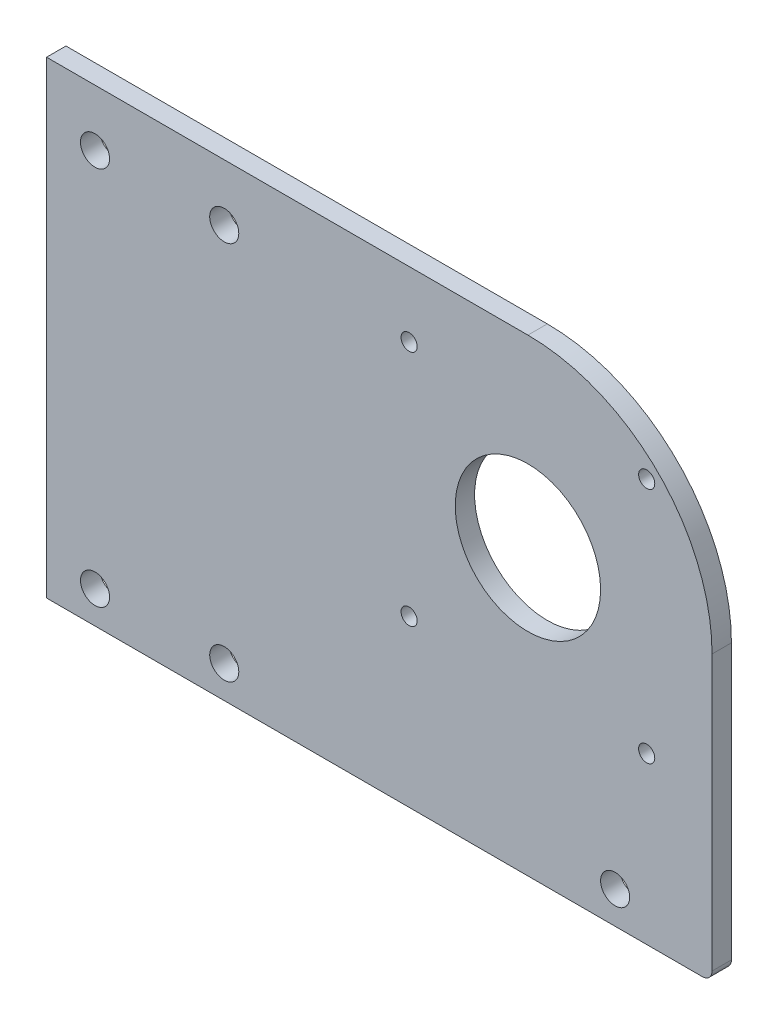
SolidWorks part; units mm, degrees
material "普通碳钢"
ref_plane "前视基准面" through (0, 0, 0) normal (0, 0, 1) x (1, 0, 0)
ref_plane "上视基准面" through (0, 0, 0) normal (0, 1, 0) x (1, 0, 0)
ref_plane "右视基准面" through (0, 0, 0) normal (1, 0, 0) x (0, 0, -1)
sketch "草图1" plane through (0, 0, 0) normal (0, 0, 1) x (1, 0, 0)
  line L0 (0, 72.5) -> (0, 0) construction
  line L1 (-103, 72.5) -> (103, 72.5)
  line L2 (-103, 72.5) -> (-103, -72.5)
  line L3 (-103, -72.5) -> (103, -72.5)
  line L4 (103, 72.5) -> (103, -72.5)
  line L5 (0, 0) -> (103, 0) construction
  dimension "D1" = 206
  dimension "D2" = 145
extrude "凸台-拉伸1" add sketch "草图1" along normal blind 6
sketch "草图2" plane through (0, 0, 6) normal (0, 0, 1) x (1, 0, 0)
  line L0 (103, 72.5) -> (-103, 72.5) construction
  line L1 (-103, -72.5) -> (-3, -72.5)
  line L2 (-103, -72.5) -> (-103, -7.5)
  line L3 (-103, -7.5) -> (-3, -7.5)
  line L4 (-3, -72.5) -> (-3, -7.5)
  dimension "D1" = 80
  dimension "D2" = 100
extrude "切除-拉伸1" [suppressed] cut sketch "草图2" against normal through all
sketch "草图3" plane through (0, 0, 6) normal (0, 0, 1) x (1, 0, 0)
  line L0 (103, 72.5) -> (-103, 72.5) construction
  line L1 (-103, 72.5) -> (-103, -72.5) construction
  circle A0 centre (-88, 55) radius 4.5
  circle A1 centre (-48, 55) radius 4.5
  circle A2 centre (-88, -62.5) radius 4.5
  circle A3 centre (-48, -62.5) radius 4.5
  dimension "D1" = 9
  dimension "D2" = 40
  dimension "D3" = 117.5
  dimension "D4" = 17.5
  dimension "D5" = 15
extrude "切除-拉伸2" cut sketch "草图3" against normal through all
sketch "草图4" plane through (0, 0, 6) normal (0, 0, 1) x (1, 0, 0)
  line L0 (103, 72.5) -> (-103, 72.5) construction
  line L2 (103, -72.5) -> (103, 72.5) construction
  circle A0 centre (46, 15.5) radius 22.5
  dimension "D1" = 45
  dimension "D3" = 57
  dimension "D2" = 57
extrude "切除-拉伸3" cut sketch "草图4" against normal through all
fillet "圆角1" radius 57 1 edges at (103, 72.5, 3)
fillet "圆角2" [suppressed] radius 10
fillet "圆角3" [suppressed] radius 10
sketch "草图5" plane through (0, 0, 6) normal (0, 0, 1) x (1, 0, 0)
  line L0 (46, 72.5) -> (-103, 72.5) construction
  line L1 (103, -72.5) -> (103, 15.5) construction
  circle A0 centre (88, 61) radius 2.75
  dimension "D1" = 11.5
  dimension "D2" = 5.5
  dimension "D3" = 15
extrude "切除-拉伸4" [suppressed] cut sketch "草图5" against normal through all
hole_wizard "M6 螺纹孔1" positions "草图7" profile "草图6" tap size "M6" standard "Gb" end condition through all
sketch "草图7" plane through (0, 0, 6) normal (0, 0, 1) x (1, 0, 0)
  line L0 (46, 41.9926) -> (46, 15.5) construction
  line L1 (46, 15.5) -> (88.8291, 15.5) construction
  line L3 (46, 15.5) -> (-6.8898, 68.3898) construction
  circle A0 centre (46, 15.5) radius 52 construction
  point P0 (9.2304, 52.2696)
  dimension "D1" = 104
  dimension "D2" = 45
cosmetic thread "孔螺蚊线1" parameters "D2"=6
sketch "草图6" plane through (9.2304, 52.2696, 6) normal (1, 0, 0) x (0, -1, 0)
  line L0 (0, 0) -> (0, 6)
  line L1 (0, 6) -> (2.5, 6)
  line L2 (2.5, 6) -> (2.5, 0)
  line L5 (2.5, 0) -> (0, 0)
  line L11 (0, -6.35) -> (0, 107.95) construction
  dimension "通孔螺纹孔钻头直径" = 5
  dimension "通孔螺纹孔钻头深度" = 6
pattern_circular "阵列(圆周)1" count 4 over 360 about axis through (46, 15.5, 0) along (0, 0, 1) of "M6 螺纹孔1"
sketch "草图8" plane through (0, 0, 6) normal (0, 0, 1) x (1, 0, 0)
  line L1 (103, -72.5) -> (98, -72.5)
  line L2 (103, -72.5) -> (103, -27.5)
  line L3 (103, -27.5) -> (98, -27.5)
  line L4 (98, -72.5) -> (98, -27.5)
  dimension "D1" = 5
  dimension "D2" = 45
extrude "切除-拉伸5" [suppressed] cut sketch "草图8" against normal through all
hole_wizard "M4 螺纹孔1" positions "草图10" profile "草图9" tap size "M4" standard "Iso"
sketch "草图10" [suppressed] plane through (98, 0, 0) normal (1, 0, 0) x (0, 0, -1)
  line L0 (-4, -72.5) -> (-4, -18.8406) construction
  line L1 (0, -72.5) -> (-8, -72.5) construction
  point P0 (-4, -37.5)
  point P2 (-4, -62.5)
  dimension "D1" = 10
  dimension "D2" = 25
sketch "草图9" plane through (98, -37.5, 4) normal (0, 1, 0) x (0, 0, -1)
  line L0 (0, 0) -> (0, 12.4914)
  line L1 (0, 12.4914) -> (1.65, 11.5)
  line L2 (1.65, 11.5) -> (1.65, 0)
  line L5 (1.65, 0) -> (0, 0)
  line L10 (0, 12.4914) -> (-1.65, 11.5) construction
  line L11 (0, -6.35) -> (0, 107.95) construction
  dimension "螺纹孔钻头直径" = 3.3
  dimension "螺纹孔钻头深度" = 11.5
  dimension "导头角度" = 118
cosmetic thread "孔螺蚊线2" [suppressed] parameters "D1"=8, "D2"=4
cosmetic thread "孔螺蚊线3" [suppressed] parameters "D1"=8, "D2"=4
fillet "圆角4" [suppressed] radius 3
sketch "草图11" plane through (0, 0, 6) normal (0, 0, 1) x (1, 0, 0)
  line L0 (-103, -72.5) -> (103, -72.5) construction
  line L1 (103, -72.5) -> (103, 15.5) construction
  circle A0 centre (73, -62.5) radius 4.5
  dimension "D1" = 10
  dimension "D2" = 30
  dimension "D3" = 9
extrude "切除-拉伸6" cut sketch "草图11" against normal through all
fillet "圆角5" radius 3 1 edges at (103, -72.5, 3)
